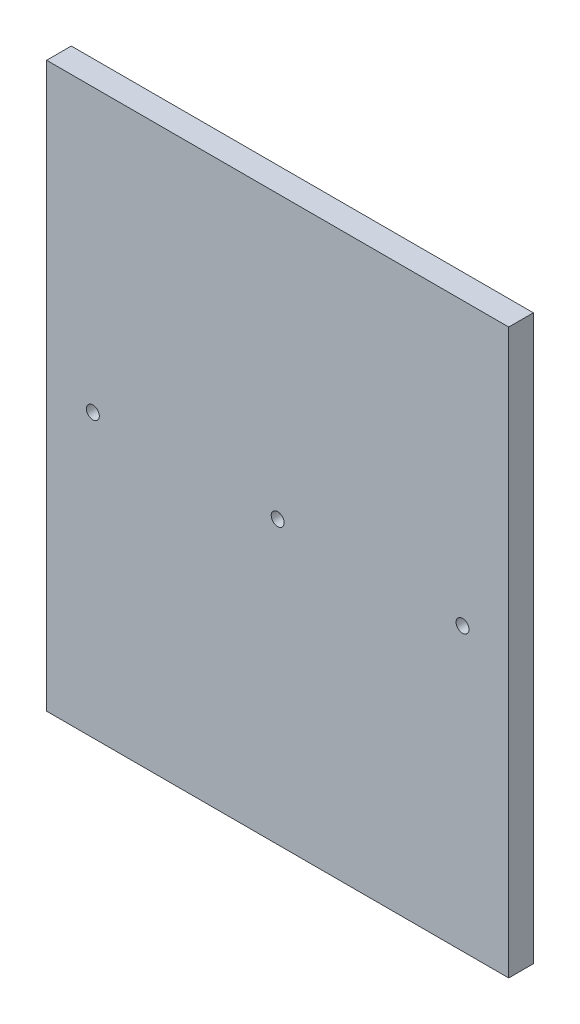
SolidWorks part; units mm, degrees
material "Q235B"
ref_plane "Front Plane" through (0, 0, 0) normal (0, 0, 1) x (1, 0, 0)
ref_plane "Top Plane" through (0, 0, 0) normal (0, 1, 0) x (1, 0, 0)
ref_plane "Right Plane" through (0, 0, 0) normal (1, 0, 0) x (0, 0, -1)
sketch "Sketch1" plane through (0, 0, 0) normal (0, 0, 1) x (1, 0, 0)
  line L1 (75, -91.5) -> (-75, -91.5)
  line L2 (75, -91.5) -> (75, 91.5)
  line L3 (75, 91.5) -> (-75, 91.5)
  line L4 (-75, -91.5) -> (-75, 91.5)
  line L5 (75, -91.5) -> (-75, 91.5) construction
  line L6 (75, 91.5) -> (-75, -91.5) construction
  point P0 (0, 0)
  dimension "D1" = 183
  dimension "D2" = 150
extrude "Boss-Extrude1" add sketch "Sketch1" along normal mid plane 8
hole_wizard "M5 Tapped Hole1" positions "Sketch2" profile "Sketch3" tap size "M5" standard "GB" end condition up to next
sketch "Sketch2" plane through (0, 0, 4) normal (0, 0, 1) x (1, 0, 0)
  line L0 (0, 29.1317) -> (0, 0) construction
  line L1 (0, 0) -> (-60, 0) construction
  point P0 (-60, 0)
  point P4 (0, 0)
  point P13 (60, 0)
  dimension "D1" = 120
sketch "Sketch3" plane through (-60, 0, 4) normal (1, 0, 0) x (0, -1, 0)
  line L0 (0, 0) -> (0, 8)
  line L1 (0, 8) -> (2.1, 8)
  line L2 (2.1, 8) -> (2.1, 0)
  line L5 (2.1, 0) -> (0, 0)
  line L11 (0, -6.35) -> (0, 107.95) construction
  dimension "通孔螺纹孔钻头直径" = 4.2
  dimension "通孔螺纹孔钻头深度" = 8
cosmetic thread "Hole Cosmetic Thread1"
cosmetic thread "Hole Cosmetic Thread2"
cosmetic thread "Hole Cosmetic Thread3"
